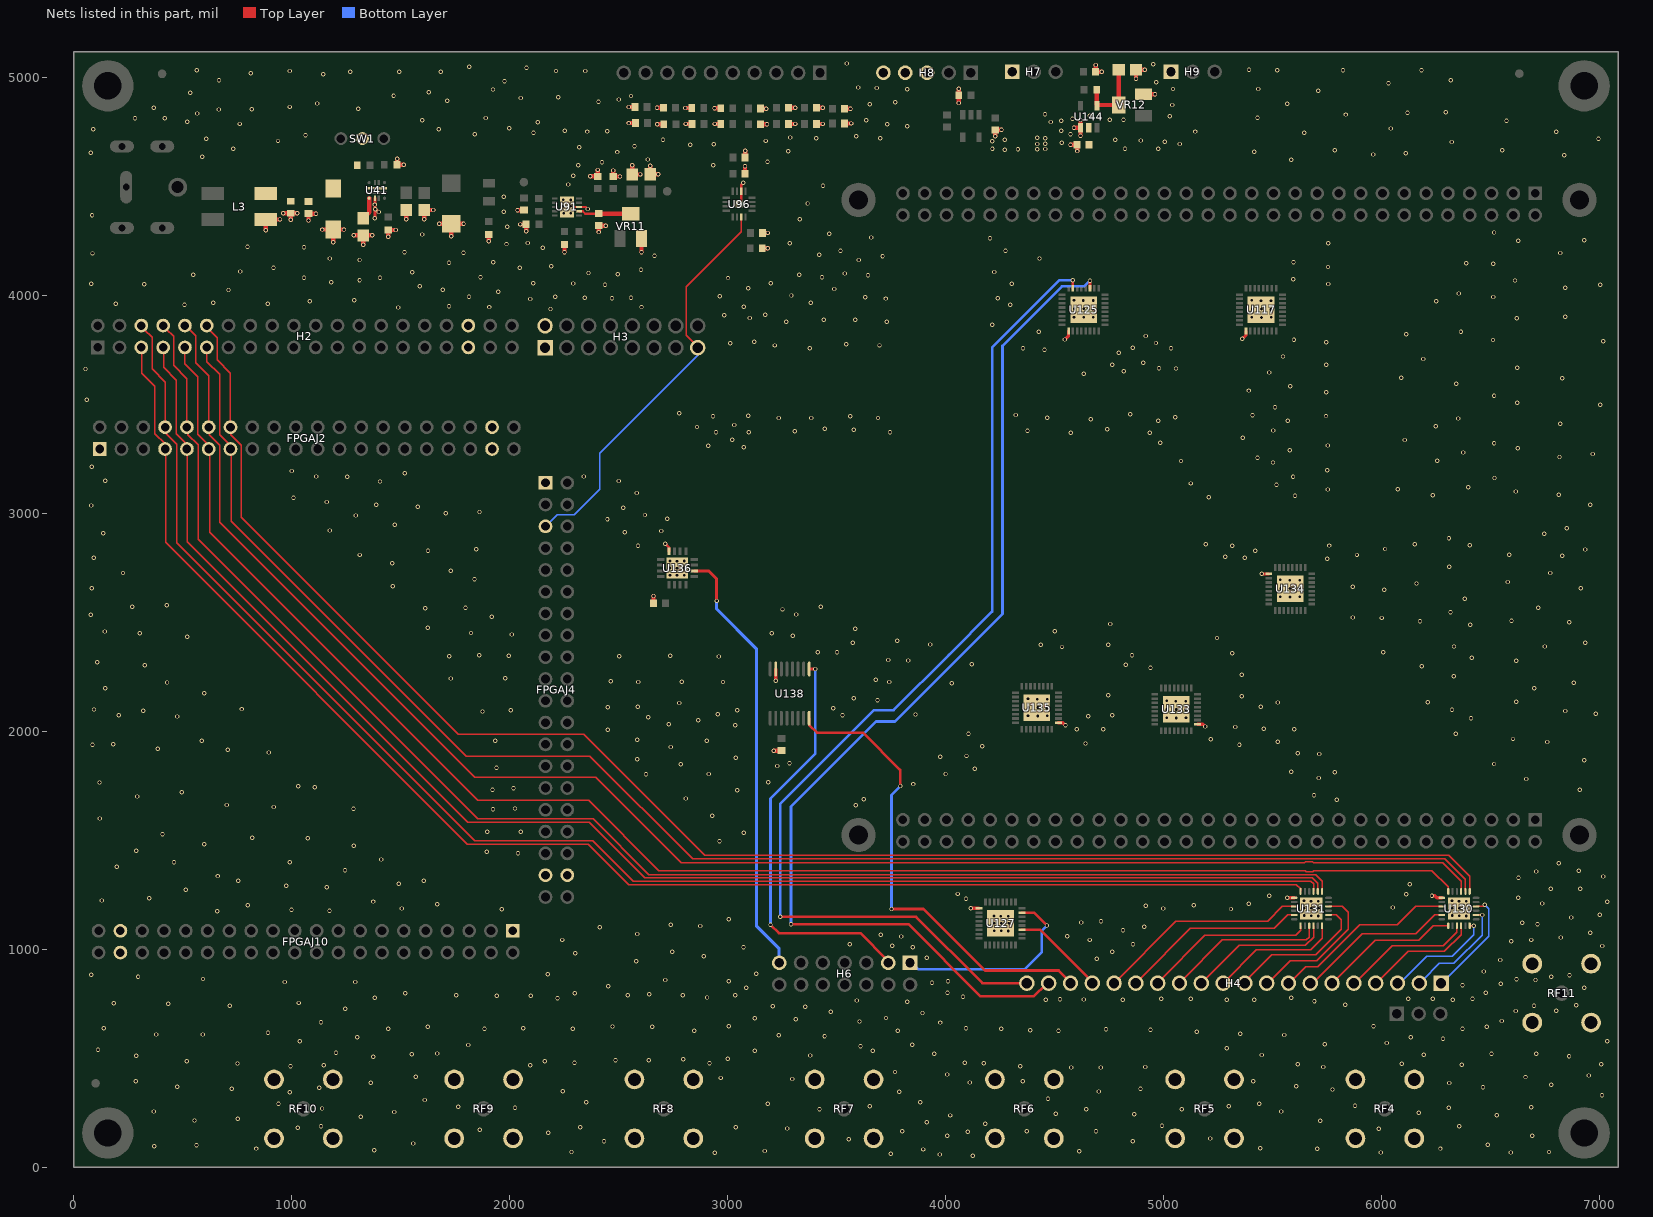
[diagram p0: the nets of this part, all layers, seen from the top]
# Altium PCB MISC82799.PcbDoc (part 3 of 5)
Units mil, origin at the board's own origin, x right, y up, seen from the top; angles counter-clockwise.
Board outline 7086.61 x 5118.11 mil, 4 copper layers (Top Layer, GND, POWER, Bottom Layer); 95 components, 232 nets, 857 pads, 1291 vias.

## Via types
v1: diameter 20, hole 12, Top Layer to Bottom Layer, 1291 vias

## Nets (pads, with @x,y where several pads share a name; then routed paths per layer and width w, separated by ;. In a path a pad name is that pad's centre, name@x,y a point inside that pad or via, vN(x,y) a via of type N, cw(c..) or ccw(c..) an arc to the next point about the centre after c; other vN are vias at no path point) (continued)
DAC_SDO: FPGAJ4.5 H3.15 U96.15 | length 1855.2
  Top Layer w6: H3.15@2859,3769 2811,3817 2811,4040 3062.85,4291.85 U96.15@3062.85,4358.94
  Bottom Layer w6: FPGAJ4.5@2175,2949 2219,2993 2296,2993 2413,3110 2413,3275 2863,3725 H3.15@2863,3760
DNW_MUX: H6.13 U136.6 | length 1996.5
  Top Layer w14: U136.6@2846.77,2736.2 2912.8,2736.2 2950,2699 v1(2950,2598)
  Bottom Layer w14: v1@2950,2596 2950,2561 3132,2379 3132,1108 3237,1003 H6.13@3237,938
DRAIN_1: H4.16 U131.3 | length 974.8
  Top Layer w6: H4.16@4771,843 H4.16@4773,845 5057,1129 5477,1129 5544.8,1196.8 U131.3@5599.26,1196.8
DRAIN_2: H4.15 U131.5 | length 828.4
  Top Layer w6: H4.15@4892,865 5123,1096 5508,1096 5569.5,1157.5 U131.5@5599.26,1157.5
DRAIN_3: H4.14 U131.7 | length 761
  Top Layer w6: H4.14@4984,858 5190,1064 5606,1064 5628.8,1086.8 U131.7@5628.8,1108.26
DRAIN_4: H4.13 U131.9 | length 714.5
  Top Layer w6: H4.13@5087,860 5270,1043 5337,1043 5655,1043 5668.2,1056.2 U131.9@5668.2,1108.26
DRAIN_5: H4.12 U131.10 | length 642.3
  Top Layer w6: H4.12@5182,853 5348,1019 5651,1019 5687.8,1055.8 U131.10@5687.8,1108.26
DRAIN_6: H4.11 U131.12 | length 586.4
  Top Layer w6: H4.11@5281,852 5426,997 5520,997 5674,997 5727.2,1050.2 U131.12@5727.2,1108.26
DRAIN_7: H4.10 U131.14 | length 644.7
  Top Layer w6: H4.10@5377,855 5497,975 5697,975 5814,1092 5814,1135 5791.5,1157.5 U131.14@5756.74,1157.5
DRAIN_8: H4.9 U131.16 | length 655.7
  Top Layer w6: H4.9@5473,840 5581,948 5702,948 5846,1092 5846,1170 5819.2,1196.8 U131.16@5756.74,1196.8
DRAIN_BOTTOM: H6.3 U138.9 | length 1988.4
  Top Layer w12: v1(3197,1112) 3235,1074 3609,1074 H6.3@3731,952 ; U138.9@3374.57,2285.82 v1(3402.83,2285.82)
  Bottom Layer w12: v1(3197,1112) 3197,1692 3402.83,1897.82 3402.83,2010 ; 3402.83,1909.18 3402.83,2010 ; v1(3402.83,2285.82) 3402.83,2010
DRAIN_DIN: FPGAJ2.7 H2.5 U131.24 | length 6803.9
  Top Layer w6: H2.5@312,3754 312,3642 372,3582 372,3366 420,3318 FPGAJ2.7@420,3295 ; FPGAJ2.7@422,3291 422,2868 1807,1483 2361,1483 2547,1297 5609,1297 5628.8,1277.2 U131.24@5628.8,1265.74
DRAIN_LEFT: H4.20 U125.31 | length 4861.7
  Top Layer w12: v1(3242,1149) 3865,1149 4169,845 H4.20@4373,845 ; U125.31@4583.78,4032.42 v1(4583.78,4069.78)
  Bottom Layer w12: v1@3241,1154 3241,1667 3671,2097 3762,2097 4016,2351 ; 4011.5,2346.5 4016,2351 ; v1(4583.78,4069.78) 4522.78,4069.78 4214,3761 4214,2549 4016,2351
DRAIN_RESET: FPGAJ2.9 H2.7 U131.20 | length 6789
  Top Layer w6: H2.7@413,3749 413,3669 471,3611 471,3365 520,3316 FPGAJ2.9@520,3295 ; FPGAJ2.9@522,3284 522,2869 1808,1583 2365,1583 2620,1328 5261,1328 ; 5257,1328 5261,1328 ; U131.20@5707.5,1265.74 5707.5,1303.5 5683,1328 5261,1328
DRAIN_RIGHT: H6.1 U127.31 | length 901.5
  Top Layer w12: U127.31@4350.42,1168.22 4405.78,1168.22 v1(4465,1109)
  Bottom Layer w12: H6.1@3853,930 3875,908 4363,908 4442,987 4442,1086 v1(4465,1109)
DRAIN_SDO: FPGAJ2.10 H2.8 U131.19 | length 6871.5
  Top Layer w6: H2.8@426,3845 460,3811 460,3678 520,3618 FPGAJ2.10@520,3395 ; FPGAJ2.10@523,3389 FPGAJ2.10@526,3386 ; FPGAJ2.10@525,3385 525,3361 571,3315 571,2882 1854,1599 2383,1599 2639,1343 5256,1343 ; 5253,1343 5256,1343 ; U131.19@5727.2,1265.74 5727.2,1312.8 5697,1343 5256,1343
DRAIN_SYNC: FPGAJ2.8 H2.6 U131.21 | length 6929.7
  Top Layer w6: H2.6@325,3842 360,3807 360,3662 420,3602 FPGAJ2.8@420,3395 ; FPGAJ2.8@425,3387 425,3365 474,3316 474,2865 1840,1499 2381,1499 2567,1313 5256,1313 ; 5252,1313 5256,1313 ; U131.21@5687.8,1265.74 5687.8,1301.2 5676,1313 5256,1313
GATE_1: H4.8 U130.3 | length 830.4
  Top Layer w6: H4.8@5587,856 5652,921 5708,921 5899,1112 6073,1112 6157.8,1196.8 U130.3@6276.26,1196.8
GATE_2: H4.7 U130.5 | length 705.1
  Top Layer w6: H4.7@5696,856 5911,1071 6157,1071 6243.5,1157.5 U130.5@6276.26,1157.5
GATE_3: H4.6 U130.7 | length 617.6
  Top Layer w6: H4.6@5790,860 5971,1041 6170,1041 6236,1107 U130.7@6304,1107 ; U130.7@6305.8,1107 U130.7@6305.8,1108.26
GATE_4: H4.5 U130.9 | length 576.5
  Top Layer w6: H4.5@5891,857 6050,1016 6284,1016 6345.2,1077.2 U130.9@6345.2,1108.26
GATE_5: H4.4 U130.10 | length 502.2
  Top Layer w6: H4.4@5990,858 6123,991 6288,991 6364.8,1067.8 U130.10@6364.8,1108.26
GATE_6: H4.3 U130.12 | length 466.5
  Top Layer w6: U130.12@6404.2,1108.26 v1(6423.26,1108.26)
  Bottom Layer w6: H4.3@6102,863 6207,968 6325,968 6423.26,1066.26 v1(6423.26,1108.26)
GATE_7: H4.2 U130.14 | length 479.8
  Top Layer w6: U130.14@6433.74,1157.5 v1(6462.5,1157.5)
  Bottom Layer w6: H4.2@6189,859 6265,935 6332,935 6462.5,1065.5 v1(6462.5,1157.5)
GATE_8: H4.1 U130.16 | length 464.8
  Top Layer w6: U130.16@6433.74,1196.8 6465.8,1196.8 v1(6474,1205)
  Bottom Layer w6: H4.1@6302,870 6492,1060 6492,1187 v1(6474,1205)
GATE_BOTTOM: H4.18 U138.8 | length 2134.3
  Top Layer w12: U138.8@3374.57,2060.18 3374.57,2029.43 3410,1994 3621,1994 3792,1823 3792,1749 v1(3793,1749) ; v1(3752,1185) 3899,1185 4181,903 4387,903 4519,903 H4.18@4562,860
  Bottom Layer w12: v1(3752,1185) 3752,1708 v1(3793,1749)
GATE_DIN: FPGAJ2.11 H2.9 U130.24 | length 7245.8
  Top Layer w6: H2.9@511,3737 511,3685 570,3626 570,3362 620,3312 FPGAJ2.11@620,3295 ; 624,3252 624,3240 ; FPGAJ2.11@624,3276 624,3240 ; 5250,1361 5254,1361 ; U130.24@6305.8,1265.74 6305.8,1286.2 6231,1361 5689,1361 5684,1356 5654,1356 5649,1361 5254,1361 ; 624,3240 624,2914 1855,1683 2363,1683 2685,1361 5254,1361
GATE_LEFT: H4.19 U125.27 | length 4997.3
  Top Layer w12: v1(3291,1115) 3830,1115 4161,784 4404,784 H4.19@4462,842 ; U125.27@4662.52,4032.42 v1(4662.52,4067.48)
  Bottom Layer w12: v1(3291,1115) 3291,1654 3682,2045 3767,2045 4261,2539 4261,3768 4534,4041 4636.05,4041 v1(4662.52,4067.48)
GATE_RESET: FPGAJ2.13 H2.11 U130.20 | length 7238.3
  Top Layer w6: H2.11@612,3742 612,3696 671,3637 671,3360 720,3311 FPGAJ2.13@720,3295 ; 724,3254 724,3224 ; FPGAJ2.13@724,3281 724,3224 ; 5242,1415 5245,1415 ; U130.20@6384.5,1265.74 6384.5,1320.5 6290,1415 5245,1415 ; 724,3224 724,2963 1801,1886 2369,1886 2840,1415 5245,1415
GATE_RIGHT: H4.17 U127.27 | length 407.2
  Top Layer w12: U127.27@4350.42,1089.48 4434.52,1089.48 H4.17@4663,861
GATE_SDO: FPGAJ2.14 H2.12 U130.19 | length 7325.2
  Top Layer w6: H2.12@622,3842 659,3805 659,3704 720,3643 FPGAJ2.14@720,3395 ; FPGAJ2.14@721,3394 721,3360 770,3311 770,2982 1765,1987 2340,1987 2896,1431 6308,1431 6404.2,1334.8 6404.2,1294 ; U130.19@6404.2,1265.74 6404.2,1294 ; 6404.2,1313.8 6404.2,1294
GATE_SYNC: FPGAJ2.12 H2.10 U130.21 | length 7381.4
  Top Layer w6: H2.10@525,3850 561,3814 561,3690 620,3631 FPGAJ2.12@620,3395 ; FPGAJ2.12@622,3391 622,3361 671,3312 671,2959 1841,1789 2395,1789 2788,1396 5251,1396 ; 5243,1396 5251,1396 ; U130.21@6364.8,1265.74 6364.8,1311.2 6280,1396 5688,1396 5682,1402 5652,1402 5646,1396 5251,1396
GND: C49.1 C50.1 C51.1 C78.1 C79.1 C216.1 C217.1 C218.1 C219.1 C329.1 C330.1 C338.1 C339.1 C340.1 C341.1 C342.1 C343.1 C344.1 C345.1 C346.1 C347.1 C348.1 C349.1 C350.1 C351.1 C352.1 C353.1 C354.1 C355.1 C356.1 C357.1 C358.1 C359.1 C360.1 C362.1 C363.1 D1.2 FPGAJ2.1 FPGAJ2.37 FPGAJ2.38 FPGAJ4.1 FPGAJ4.37 FPGAJ4.38 FPGAJ10.1 FPGAJ10.37 FPGAJ10.38 H2.35 H2.36 H3.1 H3.2 H8.3 H8.4 H8.5 H9.1 L3.3 R27.2 R28.1 R166.1 R167.1 R169.2 RF4.2 RF4.3 RF4.4 RF4.5 RF5.2 RF5.3 RF5.4 RF5.5 RF6.2 RF6.3 RF6.4 RF6.5 RF7.2 RF7.3 RF7.4 RF7.5 RF8.2 RF8.3 RF8.4 RF8.5 RF9.2 RF9.3 RF9.4 RF9.5 RF10.2 RF10.3 RF10.4 RF10.5 RF11.2 RF11.3 RF11.4 RF11.5 SW1.2 U40.1 U41.8 U42.1 U43.1 U91.8 U91.11 U96.6 U96.17 U117.9 U117.33 U125.9 U125.33 U127.9 U127.33 U130.1 U130.25 U131.1 U131.25 U133.9 U133.33 U134.9 U134.33 U135.9 U135.33 U136.12 U136.17 U138.15 U144.1 VR11.3 VR12.3 | length 3374.2
  Top Layer w10: U91.11@2293,4405 U91.8@2318.57,4405 2349,4405 v1(2358,4396)
  Top Layer w12: U96.17@3057,4429 3062.85,4434.85 U96.6@3062.85,4477.05 3062.85,4506.85 v1(3072,4516)
  Top Layer w13: v1(1382.14,4353.14) v1@1382.14,4400 ; v1(1382.14,4416.14) 1382.14,4431 ; U41.8@1382.14,4445.37 1382.14,4431 ; v1(1400,4382.14) v1@1382.14,4400 ; v1@1382.14,4400 1382.14,4431
  Top Layer w14: v1(2715,2860) 2731.61,2843.39 U136.12@2731.61,2825.77 ; v1(3221.02,2231.98) U138.15@3221.02,2285.82
  Top Layer w15: v1(4116.1,1187.9) U127.9@4153.58,1187.9 ; U135.9@4517.42,2039.1 4537.9,2039.1 v1(4550,2027) ; v1(4547,3797) 4564.1,3814.1 U125.9@4564.1,3835.57 ; U133.9@5156.42,2032.1 5180.9,2032.1 v1(5191,2022) ; v1(5361,3800) 5378.1,3817.1 U117.9@5378.1,3835.57 ; v1(5451.1,2721.9) U134.9@5482.58,2721.9 ; v1(5567.8,1236.2) U131.1@5599.26,1236.2 ; v1(6231,1246) 6244,1246 6253.8,1236.2 U130.1@6276.26,1236.2
  Top Layer w20: v1(882.05,4298.05) L3.3@882.05,4347.94 v1(946.94,4347.94) ; v1(962.44,4376.44) C49.1@997,4376.44 ; v1(997,4346) C49.1@997,4376.44 ; v1(1026.56,4376.44) C49.1@997,4376.44 ; v1(1078,4343) C50.1@1078,4374.44 v1(1112.44,4374.44) ; v1(1140.51,4301.51) U40.1@1191,4301.51 ; v1(1191,4243) U40.1@1191,4301.51 ; v1(1240.49,4301.51) U40.1@1191,4301.51 ; v1(1284.63,4274.63) C51.1@1329,4274.63 ; v1(1329,4232) C51.1@1329,4274.63 ; v1(1369.63,4274.63) C51.1@1329,4274.63 ; v1(1443,4269) R27.2@1443,4299.34 v1(1478.66,4299.34) ; v1(1484.66,4626.66) R169.2@1484.66,4598 v1(1515,4598) ; v1(1526,4348) U43.1@1526,4391.63 ; v1(1608.25,4349.25) U42.1@1608.25,4391.19 v1(1649.81,4391.19) ; v1(1676.94,4328.06) D1.2@1733,4328.06 ; v1(1733,4271) D1.2@1733,4328.06 ; v1(1789.06,4328.06) D1.2@1733,4328.06 ; v1(1905,4248) R28.1@1905,4278.34 ; v1(2036.56,4390.44) C218.1@2066,4390.44 ; v1(2049,4325) R167.1@2076.34,4325 v1(2076.34,4294.34) ; v1(2252,4198) R166.1@2252,4232.34 ; v1(2369.56,4545.56) C217.1@2405,4545.56 v1(2405,4575) ; v1(2409,4290) C219.1@2409,4319.44 v1(2441.44,4319.44) ; v1(2475.61,4572.61) C216.1@2475.61,4544.69 v1(2506.69,4544.69) ; v1(2546,4790) C356.1@2577.59,4790 ; v1(2546.89,4863.89) C357.1@2575.83,4863.89 ; v1(2562.12,4597.12) C329.1@2562.12,4554.37 v1(2600.37,4554.37) ; v1(2605.21,4197.79) VR11.3@2605.21,4259.92 ; v1(2645,4595) C330.1@2645,4555.37 v1(2682.37,4555.37) ; C340.1@2660.44,2587 v1(2660.44,2620.44) ; v1(2676.11,4859.89) C354.1@2706.59,4859.89 ; v1(2677,4785) C355.1@2707.59,4785 ; v1(2806,4859) C352.1@2835.59,4859 ; v1(2808,4786) C353.1@2836.59,4786 ; v1(2940,4858) C350.1@2968.59,4858 ; v1(2942,4786) C351.1@2968.59,4786 ; C79.1@3079.8,4557.36 v1(3079.8,4591.8) ; C78.1@3080.57,4632 v1(3080.57,4662.57) ; C348.1@3151.23,4856.31 v1(3177.69,4856.31) ; C349.1@3151.71,4785 v1(3181,4785) ; C338.1@3159.06,4216.36 v1(3184.64,4216.36) ; C339.1@3159.57,4286 v1(3185,4286) ; v1(3212.56,1911.44) C341.1@3247,1911.44 ; C347.1@3279.71,4786 v1(3310,4786) ; C346.1@3279.72,4860.31 v1(3309.69,4860.31) ; C345.1@3407.71,4786 v1(3437,4786) ; C344.1@3407.71,4860 v1(3436,4860) ; C342.1@3535.71,4856 v1(3564,4856) ; C343.1@3535.95,4788.31 v1(3566.69,4788.31) ; v1(4060.77,4882.23) C362.1@4060.77,4918.13 v1(4060.77,4947.23) ; v1(4227.33,4729.67) C363.1@4227.33,4758.57 v1(4256.57,4758.57) ; v1(4573,4691) C358.1@4603.44,4691 v1(4603.44,4661.56) ; v1(4589.18,4767.82) U144.1@4619.16,4767.82 ; v1(4619.16,4732.16) U144.1@4619.16,4767.82 ; v1(4619.16,4803.84) U144.1@4619.16,4767.82 ; v1(4688.56,5056.56) C359.1@4688.56,5025 v1(4717,5025) ; v1(4873.37,4993.63) C360.1@4873.37,5034 v1(4914,5034) ; VR12.3@4908.08,4922.21 v1(4960.79,4922.21)
  other v1: 4124,53 3974,59 3748,63 2941,66 5996,68 6592,68 2284,70 6768,70 4613,74 3171,75 1379,79 3897,82 5705,85 838,86 6270,86 5444,88 371,97 564,101 6487,103 1559,109 2433,120 4859,120 3556,128 5214,132 4008,144 6691,145 2177,158 4102,163 3802,165 4372,165 4690,166 1863,173 5987,177 3274,178 1029,182 2325,184 3038,184 6356,188 1135,189 4993,191 4182,200 3913,207 5718,213 555,215 754,223 1317,232 4021,238 6529,239 4865,243 4506,245 6171,250 1471,254 368,256 5540,256 3422,266 4646,267 5084,267 1140,270 2025,274 6308,274 6686,276 1764,278 3653,280 5299,280 5878,283 940,292 3185,292 5439,292 2352,298 3884,299 1611,309 4470,315 7011,331 992,344 3787,346 4703,348 2244,349 5775,357 726,361 4894,361 1127,365 6465,368 476,370 5608,372 6778,379 6310,387 1364,388 4111,389 285,394 4354,395 5411,395 3296,405 2968,410 6660,414 1569,416 6950,421 4007,426 3768,437 4576,458 4712,458 4916,460 5733,460 995,464 4343,464 1147,469 2095,469 6367,470 5615,473 7008,473 6092,475 752,476 2917,478 4175,478 4088,479 2298,480 520,486 2161,486 2486,491 2639,491 2797,495 3001,498 1375,508 6860,509 287,511 3380,513 5451,515 6194,517 1552,519 3948,521 6504,521 6710,521 1668,522 1204,526 3125,534 3666,535 112,539 5290,546 3610,555 1811,561 3848,562 5740,565 6023,570 1037,578 7035,579 6282,590 1302,596 6134,597 3445,601 3235,606 5553,607 379,609 592,609 5352,612 892,618 5152,622 2847,627 3781,627 4518,627 4389,628 4940,631 4736,633 1444,635 1885,635 4256,635 6371,635 2290,636 139,638 2063,638 4094,638 1624,644 2654,644 6483,644 2472,646 3005,647 5963,647 3976,664 1135,666 3605,669 6551,671 3313,680 3124,683 3727,685 3894,708 3474,713 6616,717 6802,719 1247,727 3356,736 3208,739 717,741 6699,741 6893,743 5834,745 434,750 185,752 1033,754 3825,760 5692,761 3592,765 4460,769 4813,769 5290,769 5416,769 6327,769 4634,770 4525,771 6123,773 6235,773 4989,774 5124,774 6417,774 2220,776 1381,778 5586,778 2906,779 4080,782 1942,787 2098,787 1756,789 2543,789 2794,789 3036,789 2641,794 1521,798 2299,798 4009,800 6478,800 3086,824 6930,824 2453,830 6371,835 6546,842 3938,847 969,850 1293,850 3006,853 4011,854 2715,859 6706,859 6619,863 594,864 296,874 6779,874 6862,881 81,883 2175,886 3131,888 6469,898 2582,945 6544,951 4693,956 3913,962 2891,968 2301,982 2746,988 4764,988 3073,1009 3849,1009 7013,1015 3756,1017 3560,1023 4860,1024 6594,1037 2242,1043 4661,1043 6687,1043 6822,1054 3797,1059 4558,1060 3703,1066 2586,1070 6958,1076 4288,1084 4255,1085 4223,1086 4814,1088 2414,1101 4911,1103 2875,1107 2740,1113 6715,1115 4255,1119 4223,1120 4289,1120 6645,1122 4622,1123 4713,1128 3006,1138 6870,1146 4254,1152 4287,1152 4222,1153 5710,1153 6389,1153 5677,1154 6356,1154 5645,1155 6324,1155 7000,1159 660,1174 1174,1177 1000,1182 1964,1183 5309,1185 1506,1187 4998,1187 5677,1188 6356,1188 5645,1189 5711,1189 6324,1189 6390,1189 6051,1192 4918,1199 799,1202 5139,1202 1669,1207 5391,1209 6737,1210 7035,1218 1374,1219 5676,1221 5709,1221 6355,1221 6388,1221 5644,1222 6323,1222 129,1224 4094,1232 347,1234 6627,1237 5485,1246 6114,1252 4056,1254 514,1273 6776,1278 6911,1278 1161,1285 975,1291 6129,1299 1491,1301 756,1314 1607,1314 6628,1328 7016,1334 662,1336 6710,1357 6905,1360 1245,1363 198,1378 6813,1394 461,1400 992,1400 1411,1412 2039,1441 1896,1447 288,1452 1285,1475 600,1482 2963,1495 1075,1510 819,1512 408,1527 3075,1534 1897,1540 2051,1540 121,1600 2930,1613 1924,1642 1284,1645 2025,1646 918,1653 3588,1661 702,1662 5794,1686 3624,1689 2808,1692 293,1701 5690,1707 496,1720 3044,1729 1922,1732 6909,1732 2018,1738 1107,1743 1030,1748 3851,1758 119,1765 3187,1766 6663,1781 5711,1786 2626,1803 2913,1804 4000,1804 5785,1812 5586,1814 4134,1828 1940,1832 3228,1841 2786,1849 6516,1850 3284,1854 6930,1867 2586,1872 3038,1878 3976,1883 4096,1887 5714,1896 5615,1900 895,1903 707,1916 387,1920 2740,1928 4168,1931 87,1939 5348,1939 182,1940 4642,1944 6760,1951 5523,1952 588,1956 1935,1957 2904,1957 2586,1961 5216,1964 6603,1965 4105,1988 6340,1988 2450,2007 4723,2009 4602,2010 5599,2010 5459,2012 5328,2020 3036,2027 2731,2032 2865,2051 6410,2060 5058,2061 5014,2062 5103,2062 2637,2064 476,2068 4655,2069 4422,2070 4378,2071 4467,2071 208,2073 3527,2073 4765,2073 3862,2077 2955,2078 6982,2080 1876,2091 6843,2093 320,2095 2006,2097 3044,2097 5101,2098 6323,2099 94,2100 5015,2100 5058,2100 772,2102 3485,2105 4465,2107 4379,2109 4422,2109 2450,2110 2588,2112 5446,2112 2779,2130 5523,2132 6211,2134 6617,2135 5056,2138 5102,2138 5014,2140 3688,2143 4420,2147 4466,2147 4378,2149 3579,2152 5359,2161 4747,2165 600,2174 146,2198 6701,2198 4028,2220 6882,2222 429,2224 2591,2226 2979,2226 3741,2226 2790,2227 2464,2229 3680,2237 1730,2242 1981,2244 6331,2253 5358,2259 4940,2292 6185,2299 326,2303 4826,2305 4120,2308 109,2316 6617,2323 3829,2325 3737,2327 6413,2338 2959,2343 1723,2345 2503,2345 1997,2347 2737,2347 1861,2349 4855,2349 5315,2358 6007,2362 3413,2363 3502,2363 4534,2387 6332,2389 6749,2389 4436,2397 4747,2397 3930,2398 3574,2406 6934,2406 3778,2415 5245,2428 522,2434 3299,2438 2010,2444 303,2450 3202,2450 1823,2451 143,2458 4501,2459 3585,2471 1624,2475 6406,2489 4756,2492 6861,2500 6176,2505 6596,2507 6001,2520 5867,2522 1918,2526 79,2534 3315,2536 6316,2546 3252,2559 1613,2565 1798,2566 6718,2566 270,2571 3428,2571 427,2579 6382,2608 5580,2616 5536,2617 5625,2617 6012,2650 5623,2653 5537,2655 5580,2655 84,2657 6913,2657 5867,2663 1465,2666 6160,2678 6579,2685 5578,2693 5624,2693 5536,2695 1839,2698 2768,2715 2736,2716 2802,2716 227,2726 6774,2726 1730,2737 2768,2748 2736,2749 2802,2749 6310,2755 1462,2771 2768,2780 2736,2781 2802,2781 5751,2792 92,2796 5372,2796 5283,2801 6829,2806 1313,2809 5887,2809 6586,2810 1626,2828 5421,2829 6934,2834 1848,2835 6016,2836 2589,2851 5315,2851 5760,2852 6404,2853 5193,2858 6152,2858 6309,2886 6746,2907 137,2909 2528,2913 2696,2919 1176,2921 6850,2932 1473,2947 2449,2972 2724,2975 1295,2990 2621,2992 1707,3001 1862,3006 2522,3026 1579,3030 82,3036 1389,3039 6958,3039 1162,3052 1009,3071 5207,3073 5603,3080 6235,3083 6812,3085 2584,3093 6615,3100 5753,3109 6074,3110 6397,3120 5518,3131 5125,3137 1406,3146 2501,3148 146,3150 6518,3162 1256,3167 5594,3167 1113,3169 2340,3169 1519,3184 1001,3194 5750,3197 84,3214 5502,3233 5080,3240 6255,3241 5431,3255 6816,3258 6969,3272 6374,3279 5578,3289 6625,3298 3074,3303 2912,3310 5753,3311 6516,3321 4984,3323 6106,3336 3022,3337 5363,3346 4575,3369 4936,3369 2947,3372 3098,3372 3745,3372 3309,3377 4376,3378 5503,3380 3579,3384 4742,3385 3446,3387 2860,3396 6248,3400 3031,3405 6819,3411 5570,3424 4976,3425 4666,3431 6352,3435 3235,3437 3384,3437 3690,3437 4466,3439 5053,3441 2933,3445 3563,3445 5745,3446 3095,3447 5408,3449 4322,3451 4847,3454 2778,3459 5511,3487 7003,3498 6622,3507 60,3521 6516,3539 5746,3555 5390,3563 5581,3583 6342,3594 6829,3620 6091,3621 4634,3640 5485,3646 4817,3652 55,3662 5057,3664 4979,3666 6622,3668 4765,3681 5746,3682 4907,3690 6191,3708 5548,3719 4795,3736 4454,3751 3377,3757 4355,3757 5034,3757 4859,3760 3217,3770 3697,3770 3544,3775 3012,3780 4965,3781 5746,3784 3123,3787 7017,3790 6511,3795 5598,3796 4919,3813 6114,3822 6364,3832 4428,3833 4214,3865 3269,3878 3730,3879 3585,3887 3441,3888 6620,3894 3101,3896 5449,3898 4633,3899 5405,3899 5494,3899 4589,3900 4678,3900 6843,3902 2985,3909 3173,3911 5492,3935 4676,3936 2188,3937 5406,3937 5449,3937 4590,3938 4633,3938 1489,3944 1907,3946 2605,3946 3075,3947 1722,3949 4296,3956 509,3957 891,3961 193,3962 641,3965 3381,3966 1083,3973 6250,3973 5447,3975 5493,3975 4631,3976 4677,3976 1288,3977 5405,3977 4589,3978 2095,3983 3726,3985 2470,3986 4239,3986 2557,3988 2345,3989 3631,3991 6513,3992 2209,3993 1814,3994 2964,3996 3293,3999 6354,4008 1949,4016 711,4024 1693,4025 3490,4029 3095,4032 6843,4034 1588,4042 2438,4048 7003,4048 325,4050 5755,4052 82,4053 4304,4053 2293,4054 2109,4055 3198,4056 1182,4060 6612,4068 1312,4069 5595,4073 3002,4079 1406,4080 1057,4081 1867,4083 3433,4083 3644,4092 549,4095 3329,4095 2497,4097 3538,4100 2362,4102 1554,4105 4224,4107 765,4109 2603,4117 917,4126 2047,4126 5754,4130 2191,4133 6513,4145 6389,4147 1722,4150 1926,4152 5596,4152 1312,4162 3601,4162 1175,4169 4431,4169 3711,4179 2665,4181 3420,4186 87,4192 6819,4194 1789,4195 1518,4197 3518,4204 4275,4204 2152,4218 1057,4221 798,4223 1986,4235 5756,4238 3285,4239 2083,4240 6627,4251 6930,4253 4204,4262 3659,4265 1600,4279 3466,4282 6516,4288 1990,4315 3331,4349 85,4367 2248,4376 2281,4376 1974,4384 1384,4394 2247,4408 2280,4408 3053,4419 3367,4421 2281,4437 2246,4438 1973,4452 3438,4503 2270,4508 2293,4549 2315,4597 2935,4597 2424,4611 3183,4612 5585,4621 2634,4623 590,4636 6838,4643 5962,4646 6111,4651 79,4654 2494,4657 5416,4658 3278,4661 5786,4666 6553,4666 4272,4667 4332,4670 733,4672 4215,4672 4823,4672 4975,4672 2320,4679 2573,4684 2829,4690 2937,4693 5074,4694 4533,4699 6322,4703 5006,4704 4214,4707 938,4708 3176,4708 4895,4710 2704,4713 4272,4713 4778,4714 608,4718 6995,4718 3701,4720 3407,4721 3287,4724 3590,4729 1064,4734 1841,4738 4573,4738 2110,4745 5645,4745 6801,4750 2357,4751 5145,4751 2448,4752 2253,4754 4531,4755 90,4761 1676,4762 6042,4765 1999,4766 3825,4775 3733,4785 763,4786 2130,4793 4482,4795 522,4796 6573,4800 4531,4801 1600,4803 3636,4803 4816,4805 4753,4806 4582,4809 282,4812 418,4812 1891,4813 5431,4815 4704,4819 5028,4821 4662,4823 5836,4829 4456,4831 568,4834 6119,4837 6295,4839 666,4852 817,4854 1306,4855 368,4860 992,4864 5039,4873 3653,4877 5568,4879 1118,4880 3770,4886 2408,4888 1714,4893 2501,4898 2052,4905 2224,4908 2557,4914 1468,4915 535,4929 1629,4932 5709,4939 1924,4944 3824,4945 5043,4946 5434,4946 3685,4951 3599,4953 6032,4973 4966,4977 1977,4981 6317,4986 667,4987 1146,5014 813,5018 1270,5025 1494,5025 1685,5025 992,5029 2213,5029 2348,5029 566,5033 5521,5033 5823,5033 6183,5033 5392,5035 2078,5043 1815,5048 4952,5060 3546,5063
NetC49_2: C49.2 C50.2 L3.4 R25.1 U40.2 U41.5
NetC51_2: C51.2 U41.7 | length 103.8
  Top Layer w20: C51.2@1329,4353.37 1356,4380.37 U41.7@1356,4446
NetC219_2: C219.2 U91.7 VR11.2 | length 210.6
  Top Layer w10: U91.7@2318.57,4385.31 2335.69,4385.31 2347,4374 C219.2@2404,4374
  Top Layer w20: C219.2@2409,4374.56 VR11.2@2529.44,4374.56
NetC358_2: C358.2 H7.1 U144.2
  other v1: 4421,4670 4457,4671 4421,4694 4457,4695 4458,4721 4421,4722
NetC360_2: C360.2 R170.1 U144.4 VR12.2 | length 318.3
  Top Layer w20: R170.1@4694,4933 4694,4875 4696,4873 4791,4873 4794.63,4876.63 C360.2@4794.63,5034